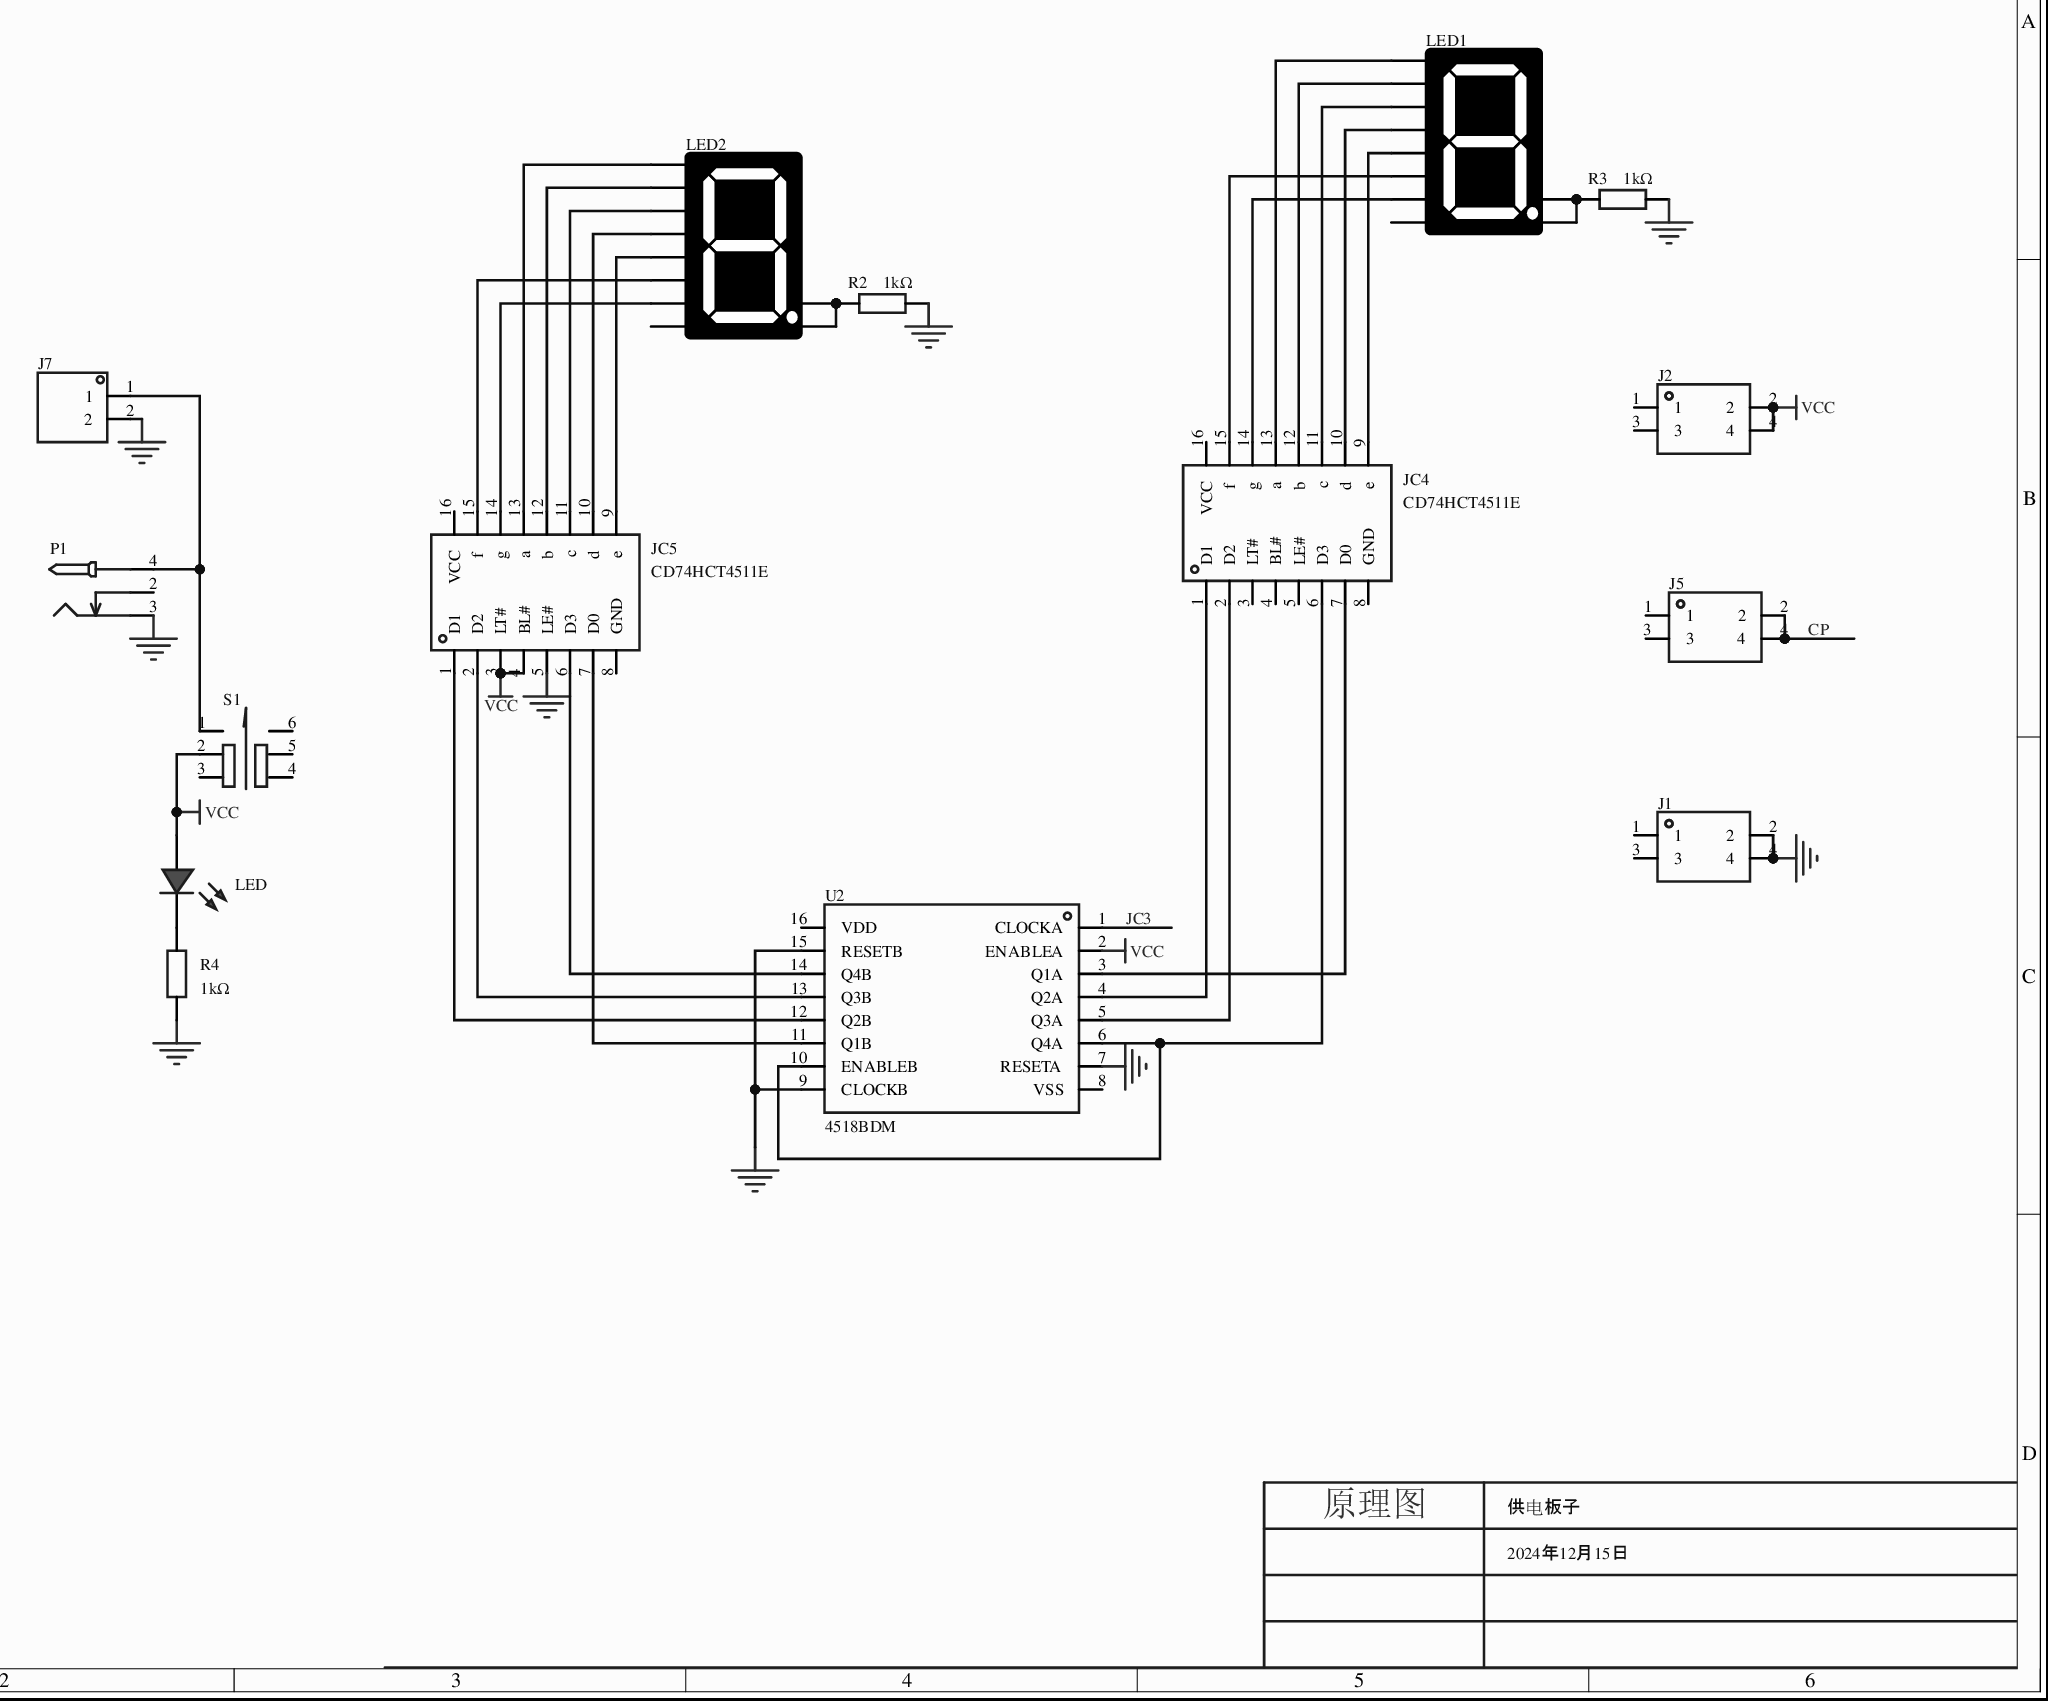
[diagram p0: MISC51364-3.schdoc]
# Altium project MISC51364-2.PrjPcb
1 sheet, 15 parts. Net scope: global (net labels, ports and power ports of the same name join across sheets).
Board file: MISC51364.pcbdoc

## Sheet MISC51364-3.schdoc
size 297 x 209 mm; Version: V1.0; @Project Name: MISC51364; @Page Count: 1; @Update Date: 2024-12-10; @Create Date: 2024-12-10; @Schematic Name: MISC51364; @Page No: 1; @Board Name: MISC51364; @Create Time: 12:48:46; @Update Time: 12:56:21

### Parts
J1  (no value)  [HDR-TH_4P-P2.54-V-M-R2-C2-S2.54-1]
J2  (no value)  [HDR-TH_4P-P2.54-V-M-R2-C2-S2.54-1]
J5  (no value)  [HDR-TH_4P-P2.54-V-M-R2-C2-S2.54-1]
J7  (no value)  [HDR-TH_2P-P2.54-V-M-1]
JC4  CD74HCT4511E  [PDIP-16_L19.3-W6.4-P2.54-LS7.94-BL]
JC5  CD74HCT4511E  [PDIP-16_L19.3-W6.4-P2.54-LS7.94-BL]
LED  (no value)  [LED-TH_5mm]
LED1  (no value)  [LED-SEG-TH_10P-L12.6-W19.0-P2.54-S15.24-BL]
LED2  (no value)  [LED-SEG-TH_10P-L12.6-W19.0-P2.54-S15.24-BL]
P1  (no value)  [DC-2.0]
R2  1kΩ  [Res_1/8W]
R3  1kΩ  [Res_1/8W]
R4  1kΩ  [Res_1/8W]
S1  自锁开关 5.8Z白灰白260G  [SW-TH_6P-L5.8-W5.8-P2.00-LS4.5-TR]  (value not drawn)
U2  4518BDM  [PDIP-16_L19.3-W6.4-P2.54-LS7.94-BL]

### Nets
GND: J1.2 J1.4 J7.2 JC5.5(LE#) P1.3 R2.2 R3.2 R4.1 U2.7(RESETA) U2.9(CLOCKB) U2.15(RESETB)
VCC: J2.2 J2.4 JC5.3(LT#) JC5.4(BL#) LED.1(C) S1.2 U2.2(ENABLEA)
CP: J5.2 J5.4
JC3: U2.1(CLOCKA)
NetJ7_1: J7.1 P1.4 S1.1
NetJC4_1: JC4.1(D1) U2.4(Q2A)
NetJC4_2: JC4.2(D2) U2.5(Q3A)
NetJC4_6: JC4.6(D3) U2.6(Q4A) U2.10(ENABLEB)
NetJC4_7: JC4.7(D0) U2.3(Q1A)
NetJC4_9: JC4.9(e) LED1.1(E)
NetJC4_10: JC4.10(d) LED1.2(D)
NetJC4_11: JC4.11(c) LED1.4(C)
NetJC4_12: JC4.12(b) LED1.6(B)
NetJC4_13: JC4.13(a) LED1.7(A)
NetJC4_14: JC4.14(g) LED1.10(G)
NetJC4_15: JC4.15(f) LED1.9(F)
NetJC5_1: JC5.1(D1) U2.12(Q2B)
NetJC5_2: JC5.2(D2) U2.13(Q3B)
NetJC5_6: JC5.6(D3) U2.14(Q4B)
NetJC5_7: JC5.7(D0) U2.11(Q1B)
NetJC5_9: JC5.9(e) LED2.1(E)
NetJC5_10: JC5.10(d) LED2.2(D)
NetJC5_11: JC5.11(c) LED2.4(C)
NetJC5_12: JC5.12(b) LED2.6(B)
NetJC5_13: JC5.13(a) LED2.7(A)
NetJC5_14: JC5.14(g) LED2.10(G)
NetJC5_15: JC5.15(f) LED2.9(F)
NetLED1_3: LED1.3(G1) LED1.8(G2) R3.1
NetLED2_3: LED2.3(G1) LED2.8(G2) R2.1
NetLED_2: LED.2(A) R4.2

Not connected (* = marked no-connect by the designer): J1 1 3; J2 1 3; J5 1 3; JC4 3(LT#) 4(BL#) 5(LE#) 8(GND) 16(VCC); JC5 8(GND) 16(VCC); LED1 5(DP); LED2 5(DP); P1 2; S1 3 4 5 6; U2 8(VSS) 16(VDD)

### Notes on the sheet
- 供电板子
- 2024年12月15日
- PERSON_A
- 原理图

### Library data of the parts
J1 J2 J5 = HDR-M_2.54_2x2: Symbol: HDR-M-2.54_2x2; ConvertToPcb: yes; ModelId: a613bc76fed24befa26ddc895095eb8f; ModelName: HDR2.54-M-LI-2x2P; ModelTransform: 200,200,0,0,0,0,0,0,-118.11; Device: HDR-M_2.54_2x2; AddInBom: yes; SupplierPart: C160338; Supplier Footprint: 插件,P=2.54mm; FootprintName: HDR-TH_4P-P2.54-V-M-R2-C2-S2.54-1
J7 = HDR-M_2.54_1x2P: Symbol: 210S-1*2P L=11.6MMGold-plated black; ConvertToPcb: yes; ModelId: 79b2e9f2d70a4d68a1b7098f27c6d4c5; ModelName: HDR-M-2.54_1x2; ModelTransform: 200,100,0,0,0,0,0,0,-118.11; Device: HDR-M_2.54_1x2P; AddInBom: yes; SupplierPart: C124375; Supplier Footprint: 插件; FootprintName: HDR-TH_2P-P2.54-V-M-1
JC4 JC5 = CD74HCT4511E: 高速 CMOS 逻辑 BCD 至 7 段锁存器/解码器/驱动器 16-PDIP -55 to 125; Manufacturer: TI(德州仪器); AddInBom: yes; ModelId: 96ff5d01b3074dd183bcbc4cd00a63de; ModelTransform: 759.841,322.44,0,0,0,0,0,0,-137.795; Symbol: CD74HCT4511E; Device: CD74HCT4511E; LCSC Part Name: CD74HCT4511E; SupplierPart: C1524048; ManufacturerPart: CD74HCT4511E; Supplier Footprint: PDIP-16; JLCPCB Part Class: 扩展库; Datasheet: https://www.ti.com/cn/lit/gpn/cd74hc4511; Supplier: LCSC; ConvertToPcb: yes; FootprintName: PDIP-16_L19.3-W6.4-P2.54-LS7.94-BL; ModelName: PDIP-16_L19.3-W6.4-P2.54-LS7.94-BL
LED = LED_TH-R_5mm: ConvertToPcb: yes; ModelId: fe9cea1bdf7642cd8d9a5077ed0e2b58; ModelName: LED-TH_BD5.9-P2.54-RD_RED; ModelTransform: 222.16,238.98,581.81,180,0,0,-6,0,-220; Symbol: LED_TH-R; Device: LED_TH-R_5mm; AddInBom: yes; FootprintName: LED-TH_5mm; Supplier Footprint: 插件
LED1 LED2 = LED_SEG_TH_0.56x1: Symbol: LED_SEG_TH_0.56*1; ConvertToPcb: yes; ModelId: 16c3aae6d39e4ecc9e744d6eeac8d57b; ModelName: LED-SEG-TH_0.56_1p; ModelTransform: 496.062,748.03,0,0,0,0,0,0,-137.795; Device: LED_SEG_TH_0.56x1; AddInBom: yes; Supplier Footprint: 插件; FootprintName: LED-SEG-TH_10P-L12.6-W19.0-P2.54-S15.24-BL
P1 = DC-005_2.0: ConvertToPcb: yes; SymbolName: DC电源接口; ModelId: f5f20b8a2308479b936ba3c2698865bb0819f05c4eef4c71ace90d822a990e87; ModelName: DC-IN-TH_DC-5520-1; ModelTransform: 372.05,551.18,582.68,90,0,0,137.8,0,-149.61; Device: DC-005_2.0; AddInBom: yes; Supplier Footprint: 插件; FootprintName: DC-2.0
R2-R4 = Res_AXIAL-1/8W: Symbol: 电阻; ConvertToPcb: yes; ModelId: b2b5ae7ae4c642178fe0039925c86a3f; ModelName: RES-TH_BD1.8-L3.2-P7.20-D0.4; ModelTransform: 282.86,66.88,253.09,0,0,0,0,0,-191; Value: 1kΩ; Device: Res_AXIAL-1/8W; AddInBom: yes; Supplier Footprint: 轴向引线; FootprintName: Res_1/8W
S1 = 自锁开关 5.8Z白灰白260G: 耐温260度; Symbol: Self-locking switch 5.8ZWhite and white260G; AddInBom: yes; ModelId: cd839ddf8c8d4e01911ba601e759d3e9; ModelTransform: 228.346,228.346,0,0,0,0,0,0,-137.795; Device: 自锁开关 5.8Z白灰白260G; LCSC Part Name: 自锁开关 5.8Z白灰白 260G  5.8*5.8mm; SupplierPart: C56857; ManufacturerPart: 自锁开关 5.8Z白灰白260G; Supplier Footprint: 插件; JLCPCB Part Class: 扩展库; Supplier: LCSC; ConvertToPcb: yes; FootprintName: SW-TH_6P-L5.8-W5.8-P2.00-LS4.5-TR; ModelName: SW-TH_6P-L5.8-W5.8-P2.00-LS4.5-TR
U2 = 4518BDM: 工作电压:5V~15V;元件数:2;每个元件位数:4;触发器类型:正边沿；负边沿;计数速率:12MHz;; Manufacturer: TI(德州仪器); AddInBom: yes; ModelId: 96ff5d01b3074dd183bcbc4cd00a63de; ModelTransform: 759.841,322.44,0,0,0,0,0,0,-137.795; Logic Type: 十进制计数器；BCD计数器; Direction: 向上计数器; Supply Voltage: 5V~15V; Number of Elements: 2; Number of Bits per Element: 4; Reset Style: 异步; Timing mode: 同步; Count Rate: 12MHz; Symbol: 4518BDM; Device: 4518BDM; LCSC Part Name: 4518BDM; SupplierPart: C3827716; ManufacturerPart: 4518BDM; Supplier Footprint: CDIP-16; Datasheet: https://atta.szlcsc.com/upload/public/pdf/source/20230920/458A25C2999F3C3D0DD9840E436CBA09.pdf; Supplier: LCSC; ConvertToPcb: yes; FootprintName: PDIP-16_L19.3-W6.4-P2.54-LS7.94-BL; ModelName: PDIP-16_L19.3-W6.4-P2.54-LS7.94-BL; Trigger Type: 正边沿；负边沿; Operating Temperature: -